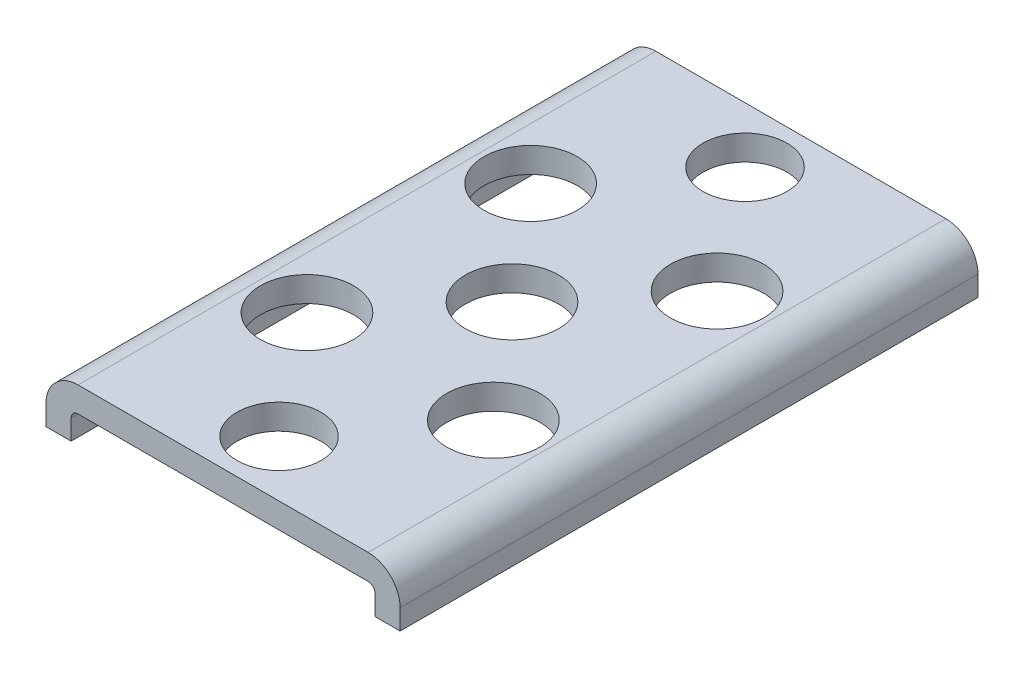
SolidWorks part; units mm, degrees
ref_plane "Front Plane" through (0, 0, 0) normal (0, 0, 1) x (1, 0, 0)
ref_plane "Top Plane" through (0, 0, 0) normal (0, 1, 0) x (1, 0, 0)
ref_plane "Right Plane" through (0, 0, 0) normal (1, 0, 0) x (0, 0, -1)
other "Configuration Table"
sketch "Sketch1" plane through (0, 0, 0) normal (0, 1, 0) x (1, 0, 0)
  line L0 (-18.9979, 14) -> (18.9979, 14)
  line L1 (18.9979, 14) -> (18.9979, 76)
  line L2 (18.9979, 76) -> (-18.9979, 76)
  line L3 (-18.9979, 76) -> (-18.9979, 14)
extrude "Boss-Extrude1" add sketch "Sketch1" against normal blind 5.5949
sketch "Sketch2" plane through (0, 0, -76) normal (0, 0, -1) x (-1, 0, 0)
  line L0 (16.2979, -5.5949) -> (16.2979, -2.7)
  line L1 (16.2979, -2.7) -> (-16.2979, -2.7)
  line L2 (-16.2979, -2.7) -> (-16.2979, -5.5949)
  line L3 (-16.2979, -5.5949) -> (16.2979, -5.5949)
extrude "Cut-Extrude1" cut sketch "Sketch2" against normal through all
hole_wizard "Ø10.0 (10) Diameter Hole1" positions "Sketch4" profile "Sketch3" hole size "Ø10.0" standard "ANSI Metric"
sketch "Sketch4" plane through (0, 0, 0) normal (0, 1, 0) x (1, 0, 0)
  point P0 (0, 45)
  point P1 (-10, 57)
  point P2 (-10, 33)
  point P3 (10, 33)
  point P4 (10, 57)
sketch "Sketch3" plane through (0, 0, -45) normal (1, 0, 0) x (0, 0, 1)
  line L0 (0, 0) -> (0, 5.5949)
  line L1 (0, 5.5949) -> (5, 5.5949)
  line L2 (5, 5.5949) -> (5, 0)
  line L5 (5, 0) -> (0, 0)
  line L11 (0, -6.35) -> (0, 107.95) construction
  dimension "通孔孔直径" = 10
  dimension "通孔孔深度" = 5.5949
hole_wizard "Ø9.0 (9) Diameter Hole1" positions "Sketch6" profile "Sketch5" hole size "Ø9.0" standard "ANSI Metric"
sketch "Sketch6" plane through (0, 0, 0) normal (0, 1, 0) x (1, 0, 0)
  point P0 (0, 70)
  point P1 (0, 20)
sketch "Sketch5" plane through (0, 0, -70) normal (1, 0, 0) x (0, 0, 1)
  line L0 (0, 0) -> (0, 5.5949)
  line L1 (0, 5.5949) -> (4.5, 5.5949)
  line L2 (4.5, 5.5949) -> (4.5, 0)
  line L5 (4.5, 0) -> (0, 0)
  line L11 (0, -6.35) -> (0, 107.95) construction
  dimension "通孔孔直径" = 9
  dimension "通孔孔深度" = 5.5949
fillet "Fillet1" radius 0.7366 2 edges at (-16.2979, -2.7, -45) (16.2979, -2.7, -45)
fillet "Fillet2" radius 3.4366 2 edges at (18.9979, 0, -45) (-18.9979, 0, -45)
